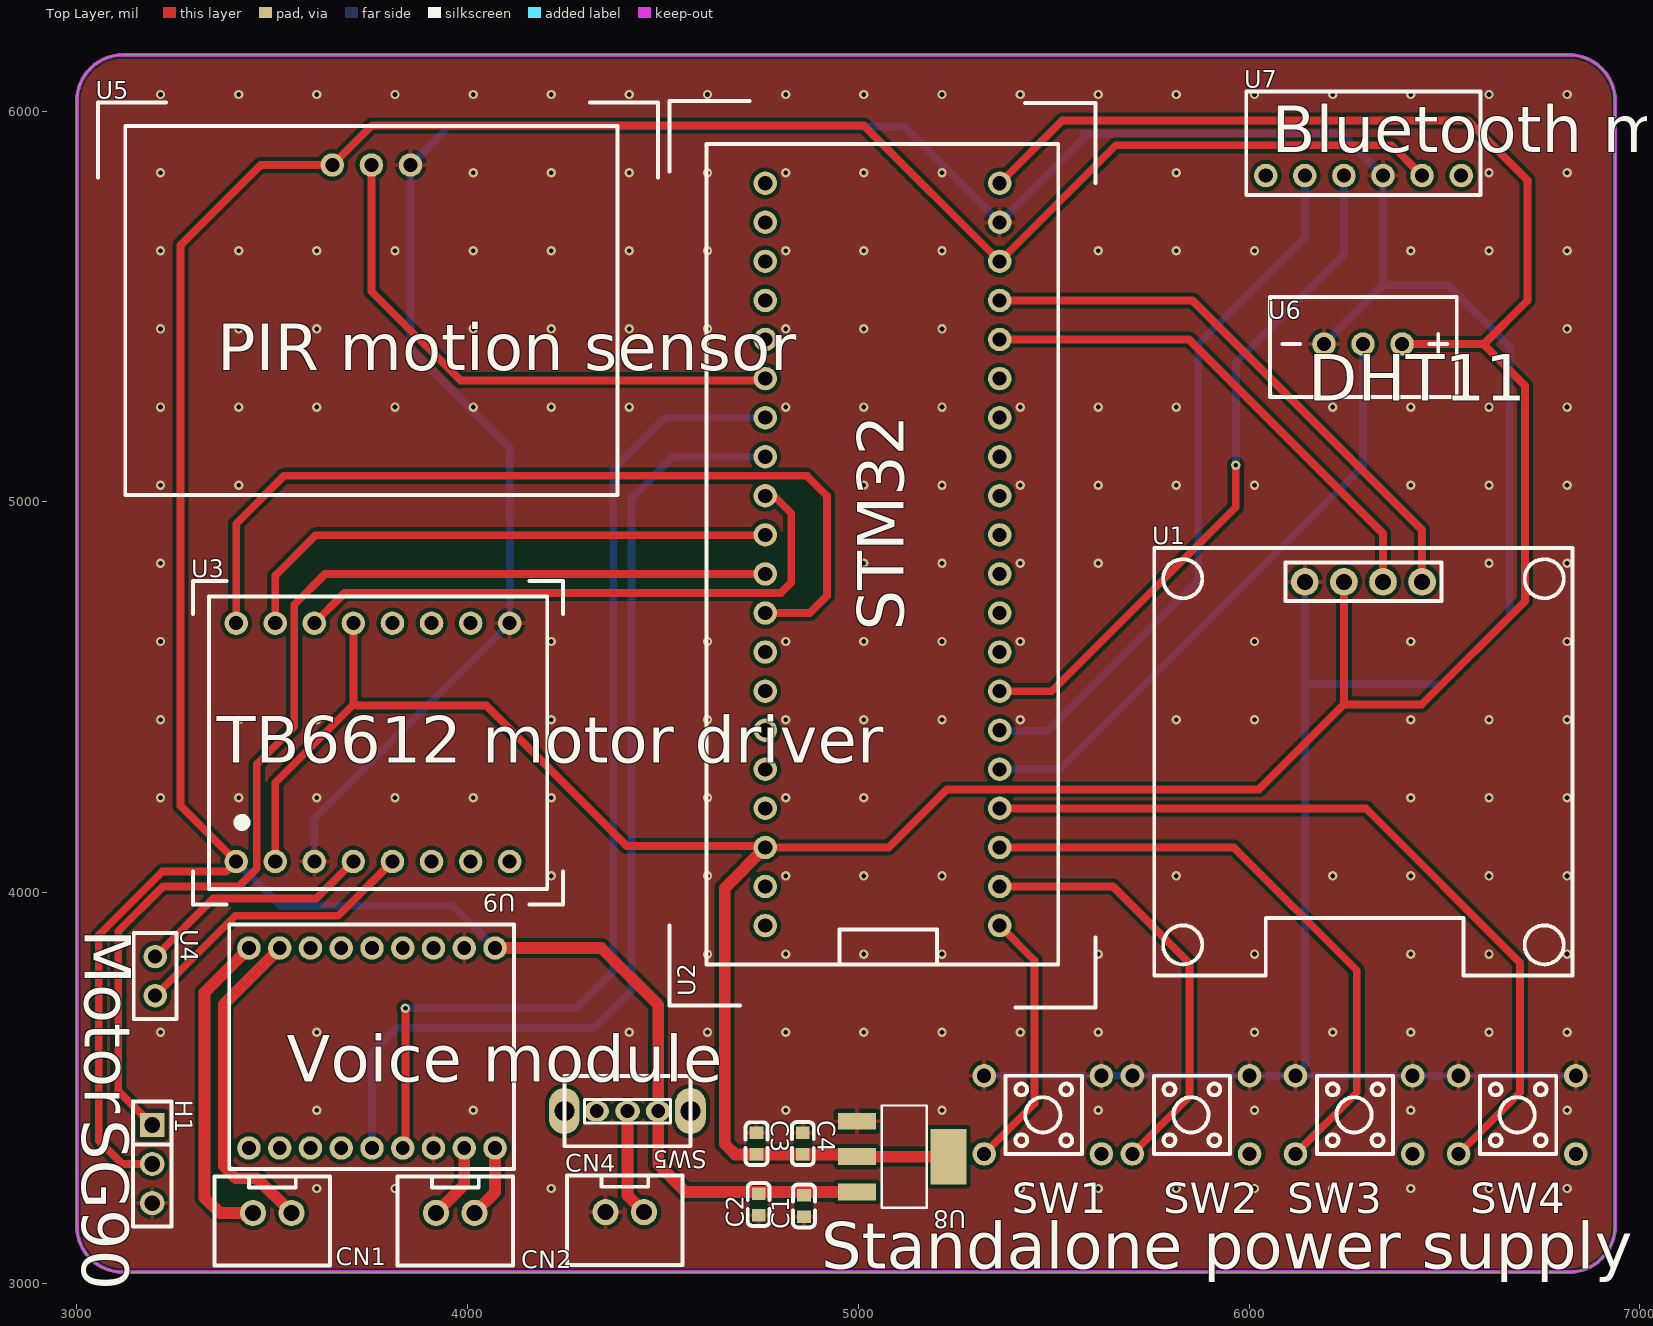
[diagram p0: Top Layer view]
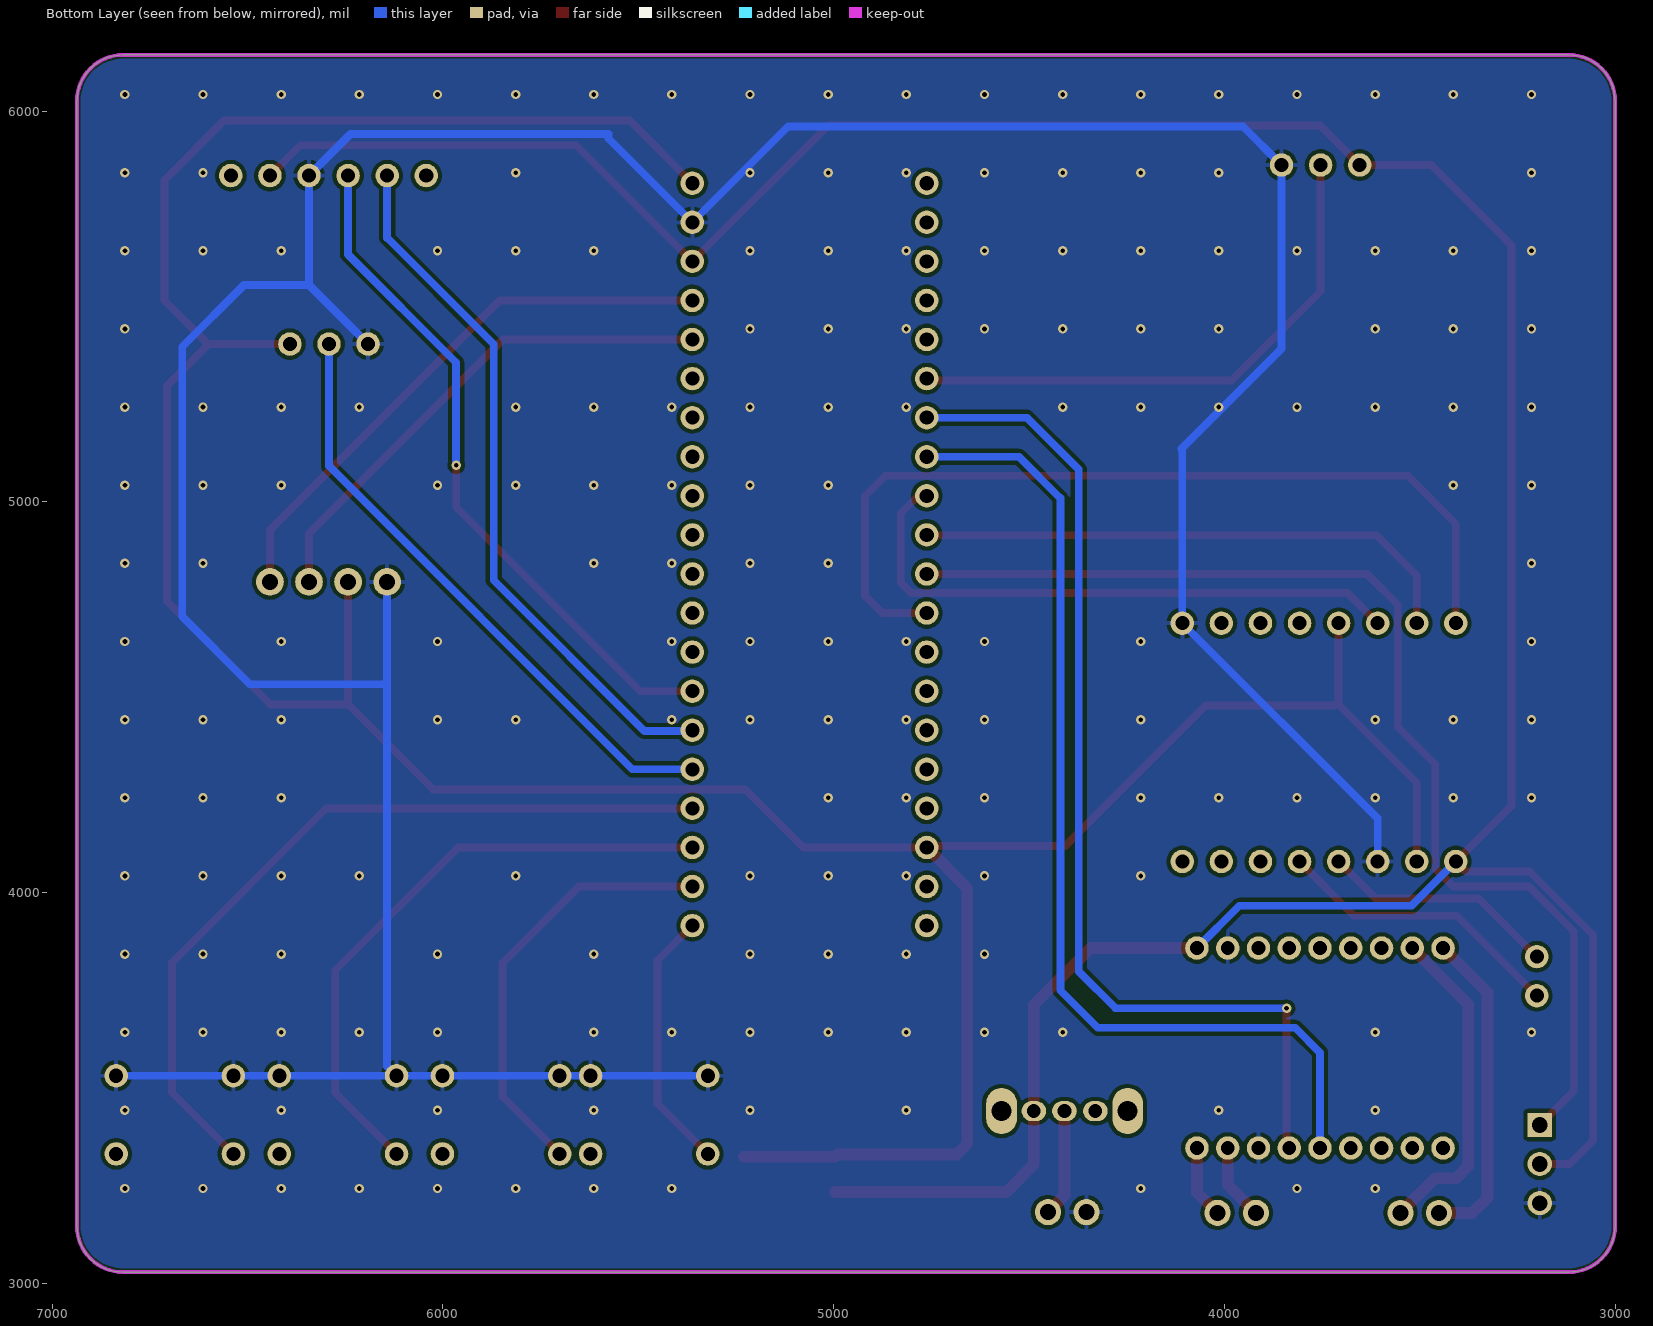
[diagram p1: Bottom Layer view, seen from below]
# Altium PCB MISC51940.pcbdoc
Units mil, origin at the board's own origin, x right, y up, seen from the top; angles counter-clockwise.
Board outline 3937.01 x 3115.51 mil, 2 copper layers (Top Layer, Bottom Layer), stack 62.206 mil thick; 22 components, 26 nets, 134 pads, 183 vias.

## Layer stack, top to bottom
Top Solder Mask Layer: solder mask 0.394, Dk 3.3
Top Layer: signal copper 1.379
Dielectric1: surface 59.449, FR4, Dk 4.5
Bottom Layer: signal copper 1.378
Bottom Solder Mask Layer: solder mask 0.394, Dk 3.3

## Board outline
3118.11,6143.8 ccw(c3118.11,6025.69) 3000,6025.69 3000,3146.4 ccw(c3118.11,3146.4) 3118.11,3028.29 6818.9,3028.29 ccw(c6818.9,3146.4) 6937.01,3146.4 6937.01,6025.69 ccw(c6818.9,6025.69) 6818.9,6143.8

## Design rules (kind name [scope] priority, off if disabled: settings)
BoardOutlineClearance copperThickness2oz_1 [All] p2 off: genericclearance=7.99 ignorepadtopadclearanceinfootprint=FALSE except(0: Arc-SplitContinuation Track-SplitContinuation SMDPad-SplitContinuation THPad-SplitContinuation Via-SplitContinuation Fill-SplitContinuation Region-SplitContinuation Poly-SplitContinuation Text-SplitContinuation Hole-SplitContinuation; 5.98: SMDPad-CutoutEdge THPad-CutoutEdge Via-CutoutEdge Fill-CutoutEdge Region-CutoutEdge Text-CutoutEdge Hole-CutoutEdge; 10: Poly-OutlineEdge Poly-CutoutEdge; 11.81: Arc-OutlineEdge Track-OutlineEdge SMDPad-OutlineEdge THPad-OutlineEdge Via-OutlineEdge Fill-OutlineEdge Region-OutlineEdge Text-OutlineEdge Hole-OutlineEdge Arc-CutoutEdge Track-CutoutEdge)
BoardOutlineClearance Plane_innerPlane_1 [All] p4 off: genericclearance=4.02 ignorepadtopadclearanceinfootprint=FALSE except(0: Arc-SplitContinuation Track-SplitContinuation SMDPad-SplitContinuation THPad-SplitContinuation Via-SplitContinuation Fill-SplitContinuation Region-SplitContinuation Poly-SplitContinuation Text-SplitContinuation Hole-SplitContinuation; 5.98: SMDPad-CutoutEdge THPad-CutoutEdge Via-CutoutEdge Fill-CutoutEdge Region-CutoutEdge Text-CutoutEdge Hole-CutoutEdge; 10: Poly-OutlineEdge Poly-CutoutEdge; 11.81: Arc-OutlineEdge Track-OutlineEdge SMDPad-OutlineEdge THPad-OutlineEdge Via-OutlineEdge Fill-OutlineEdge Region-OutlineEdge Text-OutlineEdge Hole-OutlineEdge Arc-CutoutEdge Track-CutoutEdge)
BoardOutlineClearance Copper_copperRegion_1 [All] p6 off: genericclearance=4.02 ignorepadtopadclearanceinfootprint=FALSE except(0: Arc-SplitContinuation Track-SplitContinuation SMDPad-SplitContinuation THPad-SplitContinuation Via-SplitContinuation Fill-SplitContinuation Region-SplitContinuation Poly-SplitContinuation Text-SplitContinuation Hole-SplitContinuation; 5.98: SMDPad-CutoutEdge THPad-CutoutEdge Via-CutoutEdge Fill-CutoutEdge Region-CutoutEdge Text-CutoutEdge Hole-CutoutEdge; 10: Poly-OutlineEdge Poly-CutoutEdge; 11.81: Arc-OutlineEdge Track-OutlineEdge SMDPad-OutlineEdge THPad-OutlineEdge Via-OutlineEdge Fill-OutlineEdge Region-OutlineEdge Text-OutlineEdge Hole-OutlineEdge Arc-CutoutEdge Track-CutoutEdge)
BoardOutlineClearance copperThickness1oz_1 [All] p8: genericclearance=4.02 ignorepadtopadclearanceinfootprint=FALSE except(0: Arc-SplitContinuation Track-SplitContinuation SMDPad-SplitContinuation THPad-SplitContinuation Via-SplitContinuation Fill-SplitContinuation Region-SplitContinuation Poly-SplitContinuation Text-SplitContinuation Hole-SplitContinuation; 5.98: SMDPad-CutoutEdge THPad-CutoutEdge Via-CutoutEdge Fill-CutoutEdge Region-CutoutEdge Text-CutoutEdge Hole-CutoutEdge; 10: Poly-OutlineEdge Poly-CutoutEdge; 11.81: Arc-OutlineEdge Track-OutlineEdge SMDPad-OutlineEdge THPad-OutlineEdge Via-OutlineEdge Fill-OutlineEdge Region-OutlineEdge Text-OutlineEdge Hole-OutlineEdge Arc-CutoutEdge Track-CutoutEdge)
Clearance copperThickness2oz [All] p1 off: gap=7.99 ignorepadtopadclearanceinfootprint=FALSE except(5.98: SMDPad-Track SMDPad-SMDPad THPad-Track SMDPad-THPad THPad-THPad Track-Via SMDPad-Via THPad-Via Via-Via Fill-Track Region-Track Fill-SMDPad Region-SMDPad Fill-THPad Region-THPad Fill-Via Region-Via Fill-Fill Fill-Region Region-Region Arc-Track Arc-SMDPad Arc-THPad Arc-Via Fill-Arc Region-Arc Arc-Arc Text-Track SMDPad-Text Text-THPad Text-Via Fill-Text Region-Text Arc-Text Text-Text Hole-Track Hole-SMDPad Hole-THPad Hole-Via Fill-Hole Region-Hole Hole-Arc Hole-Text; 10: Poly-Track Poly-SMDPad Poly-THPad Poly-Via Poly-Fill Poly-Region Poly-Poly Poly-Arc Poly-Text Poly-Hole)
Clearance Plane_innerPlane [All] p3 off: gap=4.02 ignorepadtopadclearanceinfootprint=FALSE except(5.98: SMDPad-Track SMDPad-SMDPad THPad-Track SMDPad-THPad THPad-THPad Track-Via SMDPad-Via THPad-Via Via-Via Fill-Track Region-Track Fill-SMDPad Region-SMDPad Fill-THPad Region-THPad Fill-Via Region-Via Fill-Fill Fill-Region Region-Region Arc-Track Arc-SMDPad Arc-THPad Arc-Via Fill-Arc Region-Arc Arc-Arc Text-Track SMDPad-Text Text-THPad Text-Via Fill-Text Region-Text Arc-Text Text-Text Hole-Track Hole-SMDPad Hole-THPad Hole-Via Fill-Hole Region-Hole Hole-Arc Hole-Text; 10: Poly-Track Poly-SMDPad Poly-THPad Poly-Via Poly-Fill Poly-Region Poly-Poly Poly-Arc Poly-Text Poly-Hole)
Clearance Copper_copperRegion [All] p5 off: gap=4.02 ignorepadtopadclearanceinfootprint=FALSE except(5.98: SMDPad-Track SMDPad-SMDPad THPad-Track SMDPad-THPad THPad-THPad Track-Via SMDPad-Via THPad-Via Via-Via Fill-Track Region-Track Fill-SMDPad Region-SMDPad Fill-THPad Region-THPad Fill-Via Region-Via Fill-Fill Fill-Region Region-Region Arc-Track Arc-SMDPad Arc-THPad Arc-Via Fill-Arc Region-Arc Arc-Arc Text-Track SMDPad-Text Text-THPad Text-Via Fill-Text Region-Text Arc-Text Text-Text Hole-Track Hole-SMDPad Hole-THPad Hole-Via Fill-Hole Region-Hole Hole-Arc Hole-Text; 10: Poly-Track Poly-SMDPad Poly-THPad Poly-Via Poly-Fill Poly-Region Poly-Poly Poly-Arc Poly-Text Poly-Hole)
Clearance copperThickness1oz [All] p7: gap=4.02 ignorepadtopadclearanceinfootprint=FALSE except(5.98: SMDPad-Track SMDPad-SMDPad THPad-Track SMDPad-THPad THPad-THPad Track-Via SMDPad-Via THPad-Via Via-Via Fill-Track Region-Track Fill-SMDPad Region-SMDPad Fill-THPad Region-THPad Fill-Via Region-Via Fill-Fill Fill-Region Region-Region Arc-Track Arc-SMDPad Arc-THPad Arc-Via Fill-Arc Region-Arc Arc-Arc Text-Track SMDPad-Text Text-THPad Text-Via Fill-Text Region-Text Arc-Text Text-Text Hole-Track Hole-SMDPad Hole-THPad Hole-Via Fill-Hole Region-Hole Hole-Arc Hole-Text; 10: Poly-Track Poly-SMDPad Poly-THPad Poly-Via Poly-Fill Poly-Region Poly-Poly Poly-Arc Poly-Text Poly-Hole)
DiffPairsRouting differentialPair [All] p1: maxlimit=6 minlimit=6 mostfreqgap=6 toplayer_minwidth=5 toplayer_prefwidth=10 toplayer_maxwidth=100 toplayer_mingap=6 toplayer_prefgap=6 toplayer_maxgap=6 bottomlayer_minwidth=5 bottomlayer_prefwidth=10 bottomlayer_maxwidth=100 bottomlayer_mingap=6 bottomlayer_prefgap=6 bottomlayer_maxgap=6 maxuncoupledlength=10
HoleToHoleClearance otherClearance [All] p1: gap=11.8 allowstackedmicrovias=TRUE
Length netLength [All] p1: minlimit=0 maxlimit=0
PasteMaskExpansion pasteMaskExpansion [All] p1: expansion=0
PlaneConnect innerPlane [All] p1: planeconnectstyle=Relief reliefexpansion=20 reliefentries=4 reliefconductorwidth=10 reliefairgap=10
PolygonConnect copperRegion [All] p1: connectstyle=Relief reliefconductorwidth=10 reliefentries=4 polygonreliefangle="90 Angle" airgapwidth=10 via.connectstyle=Relief via.reliefconductorwidth=10 via.reliefentries=4 via.polygonreliefangle="90 Angle" via.airgapwidth=10
RoutingVias viaSize [All] p1: holewidth=12.01 width=24.02 viastyle="Through Hole" minholewidth=11.81 minwidth=19.68 maxholewidth=248.03 maxwidth=393.7
SolderMaskExpansion solderMaskExpansion [IsVia] p1: expansion=-1000 istentingtop=TRUE
SolderMaskExpansion solderMaskExpansion [All] p2: expansion=2 istentingtop=FALSE
Width copperThickness2oz_2 [All] p1 off: maxlimit=100 minlimit=8 preferedwidth=10
Width copperThickness1oz_2 [All] p2: maxlimit=100 minlimit=5 preferedwidth=10

## Components (designator, comment, footprint, x,y, rotation, side; value= is the part's Value field where it differs from the comment)
C1 "100nF" C0603 4860.77,3197.68 r90 top
C2 "10uF" C0603 4745.03,3201.47 r90 top
C3 "100nF" C0603 4739.56,3357.21 r270 top
C4 "10uF" C0603 4857.99,3357.36 r270 top
CN1 "XH2.54*2P_through-hole" CONN-TH_2P-P2.50-XH2.54-2P 3500.18,3179.92 r0 top
CN2 "XH2.54*2P_through-hole" CONN-TH_2P-P2.50-XH2.54-2P 3968.5,3180.06 r0 top
CN4 "XH2.54*2P_through-hole" CONN-TH_2P-P2.50-XH2.54-2P 4402.44,3181.83 r0 top
H1 "" HDR-TH_3P-P2.54-V-F 3192.87,3305.02 r270 top
SW1 "" 按键 5322.2,3330.9 r90 top
SW2 "" 按键 5701.4,3330.9 r90 top
SW3 "" 按键 6118.9,3330.9 r90 top
SW4 "" 按键 6536.4,3330.9 r90 top
SW5 "" 拨动开关 4414.37,3440.49 r180 top
U1 "HS96L03W2C03" OLED-TH_L27.8-W27.2-P2.54_C9900033791 6292.9,4795.1 r0 top
U2 "" STM32 4761.8,3915.3 r90 top
U3 "" 电机驱动模块 3407.69,4687.3 r0 top
U4 "" 直流电机 3200.43,3835.89 r270 top
U5 "" 人体红外模块 3653.8,5861.9 r0 top
U6 "" DHT11温湿度 6191.8,5403.7 r0 top
U7 "" 蓝牙HC-08 6292.9,5834.9 r0 top
U8 "AMS1117-3.3" SOT-223-3_L6.5-W3.4-P2.30-LS7.0-BR 5113.62,3323.88 r180 top
U9 "CON2.0MM-PAD-18" CONN-TH_18P-P2.00_C9900078766 3755.32,3857.78 r180 top

## Footprints (in the part's own frame and the unit in brackets; to place one, negate y for a bottom-side part, rotate by r counter-clockwise, add the part's x,y. Pads: shape width x height; smd on the part's side, far side on the other; paste and mask are expansions set on the pad)
C0603 [mm]
  rect 0.8x0.9 smd: 1(-0.7,0) 2(0.7,0)
  silkscreen extent -1.39,-0.71 1.39,0.71
CONN-TH_2P-P2.50-XH2.54-2P [mm]
  round 1.7 hole 1.05 paste+0 mask+0.05: 1(1.25,0) 2(-1.25,0)
  silkscreen extent -3.75,-3.42 3.75,2.37
CONN-TH_18P-P2.00_C9900078766 [mil]
  round 60 hole 35.43 paste+0 mask+1.97: 1(-314.96,0.01) 2(-314.96,511.81) 3(-236.22,0.01) 4(-236.22,511.81) 5(-157.48,0.01) 6(-157.48,511.81) 9(0,0) 10(0,511.81) 11(78.74,0) 12(78.74,511.81) 13(157.48,0) 14(157.48,511.81) 15(236.22,0) 16(236.22,511.81) 17(314.96,0) 18(314.96,511.81)
  round 60 hole 35.43 copper offset -0.01,0 paste+0 mask+1.97: 7(-78.72,0.01) 8(-78.72,511.81)
  silkscreen extent -363,-60 365,565
DHT11温湿度 [mil]
  round 60 hole 36: 1(200,0) 2(100,0) 3(0,0)
  silkscreen extent -138,-135 340,120
HDR-TH_3P-P2.54-V-F [mil]
  rect 62x62 hole 40.16: 1(-100,0)
  round 62 hole 40.16: 2(0,0) 3(100,0)
  silkscreen extent -160,-49 160,49
OLED-TH_L27.8-W27.2-P2.54_C9900033791 [mm]
  round 1.8 hole 1.05 paste+0 mask+0.05: 1(-3.81,0) 2(-1.27,0) 3(1.27,0) 4(3.81,0)
  silkscreen extent -13.6,-25.6 13.6,2.2
SOT-223-3_L6.5-W3.4-P2.30-LS7.0-BR [mm]
  rect 2.5x1.1 smd: 1(2.97,-2.3) 2(2.97,0) 3(2.97,2.3)
  rect 2.34x3.6 smd: 4(-2.97,0)
  silkscreen extent -1.57,-3.33 1.37,3.33
STM32 [mil]
  round 60 hole 36: 1(0,0) 2(100,0) 3(200,0) 4(300,0) 5(400,0) 6(500,0) 7(600,0) 8(700,0) 9(800,0) 10(900,0) 11(1000,0) 12(1100,0) 13(1200,0) 14(1300,0) 15(1400,0) 16(1500,0) 17(1600,0) 18(1700,0) 19(1800,0) 20(1900,0) 21(1900,-600) 22(1800,-600) 23(1700,-600) 24(1600,-600) 25(1500,-600) 26(1400,-600) 27(1300,-600) 28(1200,-600) 29(1100,-600) 30(1000,-600) 31(900,-600) 32(800,-600) 33(700,-600) 34(600,-600) 35(500,-600) 36(400,-600) 37(300,-600) 38(200,-600) 39(100,-600) 40(0,-600)
  silkscreen extent -210,-845 2110,245
人体红外模块 [mil]
  round 60 hole 36: 1(0,0) 2(100,0) 3(200,0)
  silkscreen extent -600,-845 834,160
拨动开关 [mil]
  oval 63x51.2 hole 35.4 paste+0 mask+2: 1(-73.4,0) 2(5,0) 3(84,0)
  oval 78.7x118.1 hole 51.2 paste+0 mask+2: 4(166.7,0) 5(-156.1,0)
  silkscreen extent -156,-90 167,90
按键 [mil]
  round 60 hole 36: 1(0,0) 2(0,-300) 3(200,-300) 4(200,0)
  silkscreen extent 0,-250 200,-55
电机驱动模块 [mil]
  round 60 hole 36: 1(0,-608.03) 2(100,-608.03) 3(200,-608.03) 4(300,-608.03) 5(400,-608.03) 6(500,-608.03) 7(600,-608.03) 8(700,-608.03) 9(700,1.97) 10(600,1.97) 11(500,1.97) 12(400,1.97) 13(300,1.97) 14(200,1.97) 15(100,1.97) 16(0,1.97)
  silkscreen extent -110,-718 836,110
直流电机 [mil]
  round 60 hole 36: 1(0,0) 2(100,0)
  silkscreen extent -60,-55 160,55
蓝牙HC-08 [mil]
  round 60 hole 36: 1(-250,0) 2(-150,0) 3(-50,0) 4(50,0) 5(150,0) 6(250,0)
  silkscreen extent -300,-50 300,215

## Via types
v1: diameter 24.02, hole 12, Top Layer to Bottom Layer, 183 vias

## Nets (pads, with @x,y where several pads share a name; then routed paths per layer and width w, separated by ;. In a path a pad name is that pad's centre, name@x,y a point inside that pad or via, vN(x,y) a via of type N, cw(c..) or ccw(c..) an arc to the next point about the centre after c; other vN are vias at no path point)
$1N5250: CN4.1 SW5.2 | length 276.2
  Top Layer w30: SW5.2 4409.37,3224.12 CN4.1
+5V: C1.2 C2.2 H1.2 SW5.1 U2.23 U3.1 U5.1 U7.5 U8.3 U9.1 | length 8536.6
  Top Layer w20: H1.2 3116.18,3305.02 3056,3365.2 3056,3890.9 3218.6,4053.5 3381.92,4053.5 U3.1 3265.2,4221.76 3265.2,5656.8 3470.3,5861.9 U5.1 3755.1,5963.2 5013.9,5963.2 U2.23 5659,5912.5 6365.3,5912.5 U7.5
  Top Layer w30: U9.1 4342.73,3857.77 4487.77,3712.73 SW5.1 4487.77,3303.93 4558.37,3233.33 U8.3
  Bottom Layer w20: U3.1 3521.06,3965.9 3962.14,3965.9 U9.1
AIN1: U2.12 U3.14 | length 1526.1
  Top Layer w20: U3.14 3685.12,4766.7 4801.8,4766.7 4828.4,4793.3 4828.4,4970.4 4783.5,5015.3 U2.12
AIN2: U2.11 U3.15 | length 1419
  Top Layer w20: U3.15 3507.69,4810.99 3610.9,4914.2 4760.7,4914.2 U2.11
DATA: U2.36 U6.2 | length 1563.5
  Bottom Layer w20: U2.36 5515.2,4315.3 6291.8,5091.9 U6.2
GND: C1.1 C2.1 C3.1 C4.1 CN4.2 H1.3 SW1.3 SW1.4 SW2.3 SW2.4 SW3.3 SW3.4 SW4.3 SW4.4 U1.1 U2.22 U3.3 U3.9 U5.3 U6.3 U7.4 U8.1 U9.3 U9.6 | length 9833.2
  Bottom Layer w20: U3.3 3607.69,4189.27 U3.9 4107.69,5132.49 4110.5,5135.3 3853.8,5392 U5.3 3952.7,5960.8 5116.3,5960.8 U2.22 5576.6,5930.1 5576.6,5941.3 6236.5,5941.3 U7.4 6342.9,5554.8 ; SW1.4 SW1.3 SW2.4 SW2.3 SW3.4 ; U1.1 6142.9,4535.34 ; U6.3 6342.9,5554.8 ; SW4.3 SW4.4 SW3.3 SW3.4 ; SW3.4 6142.9,3554.9 6142.9,4535.34 ; 6142.9,4535.34 6145.24,4533 6494.3,4533 6667.5,4706.2 6667.5,5396.6 6509.3,5554.8 6342.9,5554.8
  other v1: 3614.1,3242.39 3814.1,3242.39 4214.1,3242.39 5414.1,3242.39 5614.1,3242.39 5814.1,3242.39 6014.1,3242.39 6214.1,3242.39 6414.1,3242.39 6614.1,3242.39 6814.1,3242.39 3614.1,3442.39 4014.1,3442.39 4814.1,3442.39 5214.1,3442.39 5614.1,3442.39 6014.1,3442.39 6414.1,3442.39 6814.1,3442.39 3214.1,3642.39 3614.1,3642.39 4414.1,3642.39 4614.1,3642.39 4814.1,3642.39 5014.1,3642.39 5214.1,3642.39 5414.1,3642.39 5614.1,3642.39 6014.1,3642.39 6214.1,3642.39 6414.1,3642.39 6614.1,3642.39 6814.1,3642.39 4614.1,3842.39 4814.1,3842.39 5014.1,3842.39 5214.1,3842.39 5614.1,3842.39 6014.1,3842.39 6414.1,3842.39 6614.1,3842.39 6814.1,3842.39 4214.1,4042.39 4614.1,4042.39 4814.1,4042.39 5014.1,4042.39 5214.1,4042.39 5814.1,4042.39 6214.1,4042.39 6414.1,4042.39 6614.1,4042.39 6814.1,4042.39 3214.1,4242.39 3414.1,4242.39 3614.1,4242.39 3814.1,4242.39 4014.1,4242.39 4214.1,4242.39 4614.1,4242.39 4814.1,4242.39 5014.1,4242.39 6414.1,4242.39 6614.1,4242.39 6814.1,4242.39 3214.1,4442.39 3414.1,4442.39 3614.1,4442.39 4214.1,4442.39 4614.1,4442.39 4814.1,4442.39 5014.1,4442.39 5214.1,4442.39 5414.1,4442.39 5814.1,4442.39 6014.1,4442.39 6414.1,4442.39 6614.1,4442.39 6814.1,4442.39 3214.1,4642.39 4214.1,4642.39 4614.1,4642.39 4814.1,4642.39 5014.1,4642.39 5214.1,4642.39 5414.1,4642.39 6014.1,4642.39 6414.1,4642.39 6814.1,4642.39 3214.1,4842.39 5014.1,4842.39 5214.1,4842.39 5414.1,4842.39 5614.1,4842.39 6614.1,4842.39 6814.1,4842.39 3214.1,5042.39 3414.1,5042.39 5014.1,5042.39 5214.1,5042.39 5414.1,5042.39 5614.1,5042.39 5814.1,5042.39 6014.1,5042.39 6414.1,5042.39 6614.1,5042.39 6814.1,5042.39 3214.1,5242.39 3414.1,5242.39 3614.1,5242.39 3814.1,5242.39 4014.1,5242.39 4214.1,5242.39 4414.1,5242.39 4814.1,5242.39 5014.1,5242.39 5214.1,5242.39 5414.1,5242.39 5614.1,5242.39 5814.1,5242.39 6214.1,5242.39 6414.1,5242.39 6614.1,5242.39 6814.1,5242.39 3214.1,5442.39 3414.1,5442.39 3614.1,5442.39 4014.1,5442.39 4214.1,5442.39 4414.1,5442.39 4614.1,5442.39 4814.1,5442.39 5014.1,5442.39 5214.1,5442.39 6814.1,5442.39 3214.1,5642.39 3414.1,5642.39 3614.1,5642.39 3814.1,5642.39 4014.1,5642.39 4214.1,5642.39 4414.1,5642.39 4614.1,5642.39 4814.1,5642.39 5014.1,5642.39 5214.1,5642.39 5614.1,5642.39 5814.1,5642.39 6014.1,5642.39 6414.1,5642.39 6614.1,5642.39 6814.1,5642.39 3214.1,5842.39 4014.1,5842.39 4214.1,5842.39 4414.1,5842.39 4614.1,5842.39 4814.1,5842.39 5014.1,5842.39 5214.1,5842.39 5814.1,5842.39 6614.1,5842.39 6814.1,5842.39 3214.1,6042.39 3414.1,6042.39 3614.1,6042.39 3814.1,6042.39 4014.1,6042.39 4214.1,6042.39 4414.1,6042.39 4614.1,6042.39 4814.1,6042.39 5014.1,6042.39 5214.1,6042.39 5414.1,6042.39 5614.1,6042.39 5814.1,6042.39 6014.1,6042.39 6214.1,6042.39 6414.1,6042.39 6614.1,6042.39 6814.1,6042.39
H+: U3.4 U4.1 | length 608.1
  Top Layer w20: U4.1 3348.95,3984.4 3612.82,3984.4 U3.4
KEY1: SW1.1 U2.40 | length 674.4
  Top Layer w20: SW1.1 5450.6,3459.3 5450.6,3826.5 U2.40
KEY2: SW2.1 U2.39 | length 1115.8
  Top Layer w20: U2.39 5651.7,4015.3 5847.3,3819.7 5847.3,3476.8 SW2.1
KEY3: SW3.1 U2.38 | length 1579
  Top Layer w20: U2.38 5961.3,4115.3 6275.6,3801 6275.6,3487.6 SW3.1
KEY4: SW4.1 U2.37 | length 2049.9
  Top Layer w20: U2.37 6299,4215.3 6693.3,3821 6693.3,3487.8 SW4.1
L-: U3.5 U4.2 | length 749.5
  Top Layer w20: U4.2 3405.15,3940.6 3669.02,3940.6 U3.5
MIC+: CN1.1 U9.15 | length 840.6
  Top Layer w30: U9.15 3375.6,3714.28 3375.6,3300.2 3406.9,3268.9 3460.41,3268.9 CN1.1
MIC-: CN1.2 U9.17 | length 826.7
  Top Layer w30: U9.17 3326.5,3743.92 3326.5,3218.8 3365.38,3179.92 CN1.2
OUT: U2.15 U5.2 | length 1427.4
  Top Layer w20: U5.2 3753.8,5538.8 3981.8,5310.8 4757.3,5310.8 U2.15
PA2: U2.14 U9.8 | length 2660.1
  Top Layer w20: U9.8 3840.9,3352.82 v1(3840.9,3703.6)
  Bottom Layer w20: v1(3840.9,3703.6) 4278.4,3703.6 4372.6,3797.8 4372.6,5082.5 4505.4,5215.3 U2.14
PA3: U2.13 U9.10 | length 2620.2
  Bottom Layer w20: U9.10 3755.32,3590.01 3818.9,3653.6 4323.8,3653.6 4419.8,3749.6 4419.8,5009.3 4525.8,5115.3 U2.13
PA9: U2.35 U7.2 | length 1818.1
  Bottom Layer w20: U2.35 5364.1,4413 5484.2,4413 5870.3,4799.1 5870.3,5402.9 6142.9,5675.5 U7.2
PA10: U2.34 U7.3 | length 1762.6
  Top Layer w20: U2.34 5495.1,4515.3 5965.9,4986.1 v1(5965.9,5093.4)
  Bottom Layer w20: v1(5965.9,5093.4) 5966.3,5093.8 5966.3,5356.2 6242.9,5632.8 U7.3
PWM: H1.1 U2.10 | length 2905.7
  Top Layer w20: H1.1 3105.9,3491.99 3105.9,3900.6 3220.6,4015.3 3414.08,4015.3 3460.3,4061.52 3460.3,4328.5 3556.2,4424.4 3556.2,4736.6 3634.9,4815.3 U2.10
PWMA: U2.9 U3.16 | length 2270.6
  Top Layer w20: U3.16 3407.69,4943.99 3530.2,5066.5 4868.3,5066.5 4919.5,5015.3 4919.5,4759 4875.8,4715.3 U2.9
SCL: U1.3 U2.25 | length 1310.6
  Top Layer w20: U2.25 5846.6,5415.3 6342.9,4919 U1.3
SDA: U1.4 U2.24 | length 1457.2
  Top Layer w20: U2.24 5855.4,5515.3 6442.9,4927.8 U1.4
SPK+: CN2.1 U9.2 | length 187.7
  Top Layer w30: CN2.1 4070.28,3232.62 U9.2
SPK-: CN2.2 U9.4 | length 195.8
  Top Layer w30: CN2.2 3991.53,3252.31 U9.4
VCC: C3.2 C4.2 U1.2 U2.3 U2.21 U3.2 U3.13 U6.1 U8.2 U8.4 | length 8666.6
  Top Layer w20: U3.2 3507.69,4280.49 3707.69,4480.49 3707.69,4488.71 ; U3.13 3707.69,4488.71 ; U2.21 5522.2,5975.7 6560.3,5975.7 6712.4,5823.6 6712.4,5514.7 6601.4,5403.7 6599.8,5403.7 ; U1.2 6242.9,4481.4 ; U6.1 6599.8,5403.7 ; 3707.69,4488.71 3718,4478.4 4047.6,4478.4 4407.1,4118.9 4758.2,4118.9 U2.3 5077.8,4115.3 5226.2,4263.7 6025.2,4263.7 6242.9,4481.4 ; 6242.9,4481.4 6441.9,4481.4 6706.2,4745.7 6706.2,5297.3 6599.8,5403.7
  Top Layer w30: U2.3 4657.9,4011.4 4657.9,3356.3 4684.55,3329.65 C3.2 4990.92,3329.65 U8.2 U8.4
pads on no net: SW1.2 SW2.2 SW3.2 SW4.2 SW5.3 SW5.4 SW5.5 U2.1 U2.2 U2.4 U2.5 U2.6 U2.7 U2.8 U2.16 U2.17 U2.18 U2.19 U2.20 U2.26 U2.27 U2.28 U2.29 U2.30 U2.31 U2.32 U2.33 U3.6 U3.7 U3.8 U3.10 U3.11 U3.12 U7.1 U7.6 U9.5 U9.7 U9.9 U9.11 U9.12 U9.13 U9.14 U9.16 U9.18

## Polygon pours and split planes (outlines as drawn)
GND on Bottom Layer (solid, remove dead copper, pour order 2): 3000.1,6160.9 3000.1,3017.1 6957.5,3017.1 6957.5,6160.9
GND on Top Layer (solid, remove dead copper, pour order 2): 3000.1,6132.84 3000.1,3000 6946.5,3000 6946.5,6132.84

## Keep-outs
Board Outline Layer:
  the board outline again, w10

## Silkscreen, mask and mechanical layers (free items; w line width, h text height)
Top Silkscreen Layer:
  text "Voice module" at 3537.7,3516.2 h120
  text "SG90" at 3014.2,3419.6 h120 r270
  text "Standalone power supply" at 4905,3036.6 h120